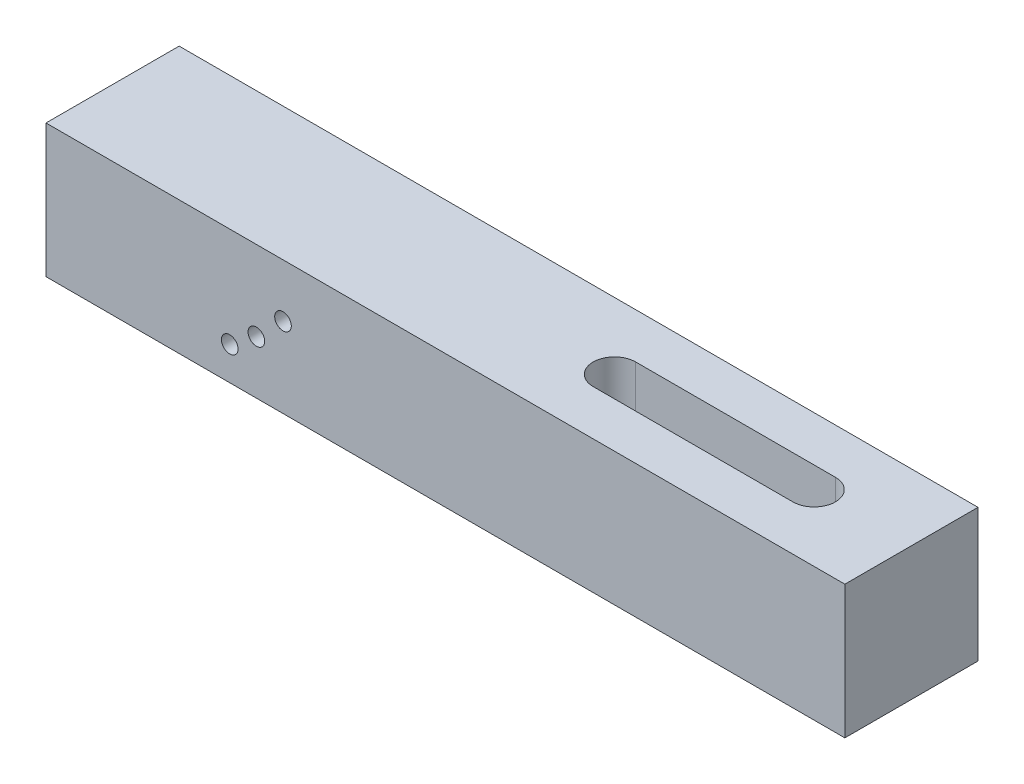
from build123d import *

# Parameters (mm, degrees)
SKETCH1_W             = 50
SKETCH1_H             = 20
BOSS_EXTRUDE1_DEPTH   = 100
SKETCH2_R             = 3
BOSS_EXTRUDE2_DEPTH   = 5
M6_TAPPED_HOLE1_D     = 5
M6_TAPPED_HOLE1_DEPTH = 15
M6_TAPPED_HOLE1_TIP   = 1.502151548
SKETCH5_W             = 20
SKETCH5_H             = 30
BOSS_EXTRUDE3_DEPTH   = 120
M3_TAPPED_HOLE1_D     = 2.5
M3_TAPPED_HOLE1_DEPTH = 7.5
M3_TAPPED_HOLE1_TIP   = 0.751075774
SKETCH8_W             = 95.008103892
SKETCH8_H             = 183.237528091
CUT_EXTRUDE1_DEPTH    = 163.249807396
CUT_EXTRUDE2_DEPTH    = 101.124921973
SKETCH10_W            = 120
SKETCH10_H            = 10
CUT_EXTRUDE3_DEPTH    = 163.249807396


with BuildPart() as part:
    # Sketch1 → Boss-Extrude1 (new body)
    with BuildSketch(Plane(origin=(0, 0, 0), x_dir=(1, 0, 0), z_dir=(0, 1, 0))):
        Rectangle(SKETCH1_W, SKETCH1_H)
    extrude(amount=BOSS_EXTRUDE1_DEPTH)

    # Sketch2 → Boss-Extrude2 (add)
    with BuildSketch(Plane.XZ):
        with Locations(Location((0, 5, 0), (0, 0, 270))):
            Circle(SKETCH2_R)
    extrude(amount=BOSS_EXTRUDE2_DEPTH)

    # M6 Tapped Hole1
    with Locations(Plane(origin=(0, 0, 0), x_dir=(-1, 0, 0), z_dir=(0, -1, 0))):
        with Locations((0, 5)):
            Hole(M6_TAPPED_HOLE1_D / 2, depth=M6_TAPPED_HOLE1_DEPTH)
            with Locations((0, 0, -(M6_TAPPED_HOLE1_DEPTH + M6_TAPPED_HOLE1_TIP / 2))):  # 118° drill point
                Cone(0, M6_TAPPED_HOLE1_D / 2, M6_TAPPED_HOLE1_TIP, mode=Mode.SUBTRACT)

    # Sketch5 → Boss-Extrude3 (add)
    with BuildSketch(Plane(origin=(25, 0, 0), x_dir=(0, 0, -1), z_dir=(1, 0, 0))):
        with Locations((0, 115)):
            Rectangle(SKETCH5_W, SKETCH5_H)
    extrude(amount=-BOSS_EXTRUDE3_DEPTH)

    # M3 Tapped Hole1
    with Locations(Plane.XY.offset(10)):
        with Locations((-63.4, 108), (-59.4, 112), (-67.4, 105)):
            Hole(M3_TAPPED_HOLE1_D / 2, depth=M3_TAPPED_HOLE1_DEPTH)
            with Locations((0, 0, -(M3_TAPPED_HOLE1_DEPTH + M3_TAPPED_HOLE1_TIP / 2))):  # 118° drill point
                Cone(0, M3_TAPPED_HOLE1_D / 2, M3_TAPPED_HOLE1_TIP, mode=Mode.SUBTRACT)

    # Sketch8 → Cut-Extrude1 (cut, through all)
    with BuildSketch(Plane.XY.offset(10)):
        with Locations((22.504051946, 8.381235954)):
            Rectangle(SKETCH8_W, SKETCH8_H)
    extrude(amount=-CUT_EXTRUDE1_DEPTH, mode=Mode.SUBTRACT)

    # Sketch9 → Cut-Extrude2 (cut, through all)
    with BuildSketch(Plane(origin=(0, 130, 0), x_dir=(1, 0, 0), z_dir=(0, 1, 0))):
        with BuildLine():
            Line((10.388294344, -3.2), (-19.611705656, -3.2))
            ThreePointArc((-19.611705656, -3.2), (-22.811705656, 0), (-19.611705656, 3.2))
            Line((-19.611705656, 3.2), (10.388294344, 3.2))
            ThreePointArc((10.388294344, 3.2), (13.588294344, 0), (10.388294344, -3.2))
        make_face()
    extrude(amount=-CUT_EXTRUDE2_DEPTH, mode=Mode.SUBTRACT)

    # Sketch10 → Cut-Extrude3 (cut, through all)
    with BuildSketch(Plane.XY.offset(10)):
        with Locations((-35, 125)):
            Rectangle(SKETCH10_W, SKETCH10_H)
    extrude(amount=-CUT_EXTRUDE3_DEPTH, mode=Mode.SUBTRACT)


solid = part.part
